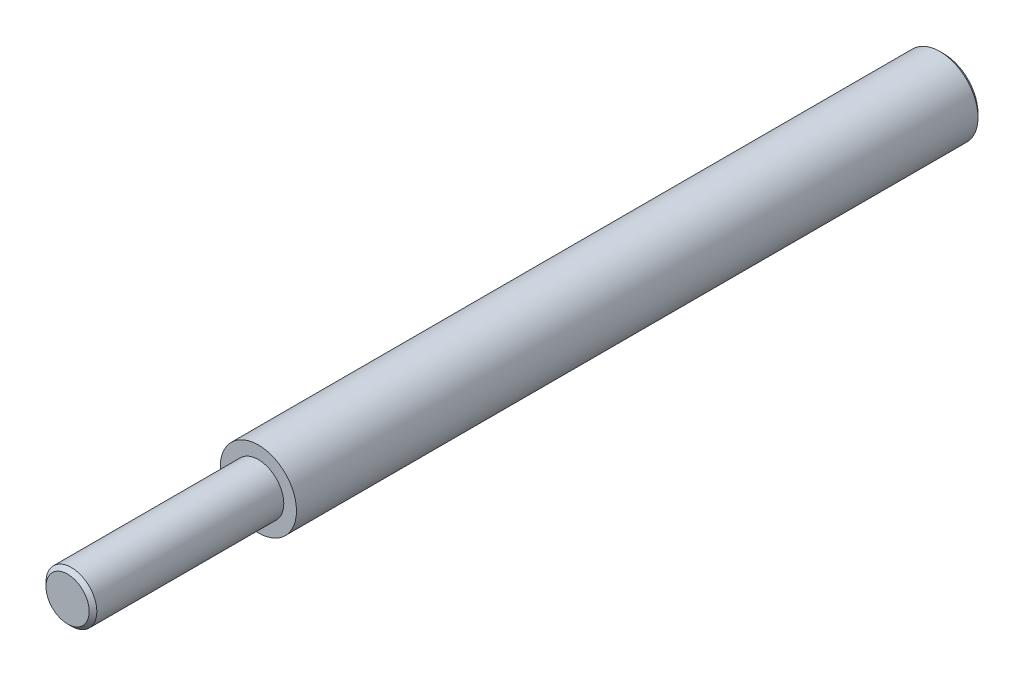
SolidWorks part; units mm, degrees
ref_plane "Front Plane" through (0, 0, 0) normal (0, 0, 1) x (1, 0, 0)
ref_plane "Top Plane" through (0, 0, 0) normal (0, 1, 0) x (1, 0, 0)
ref_plane "Right Plane" through (0, 0, 0) normal (1, 0, 0) x (0, 0, -1)
other "Configuration Table"
sketch "Sketch1" plane through (0, 0, 0) normal (0, 0, 1) x (1, 0, 0)
  circle A0 centre (0, 0) radius 5.4
  dimension "D1" = 10.8
extrude "Boss-Extrude1" add sketch "Sketch1" along normal blind 124
sketch "Sketch2" plane through (0, 0, 124) normal (0, 0, 1) x (1, 0, 0)
  circle A0 centre (0, 0) radius 3.6
  circle A1 centre (0, 0) radius 5.4 construction
  circle A2 centre (0, 0) radius 5.4
  dimension "D1" = 7.2
extrude "Cut-Extrude1" cut sketch "Sketch2" against normal blind 27
chamfer "Chamfer1" distance 0.54 angle 45 2 edges at (5.4, 0, 0) (3.6, 0, 124)
